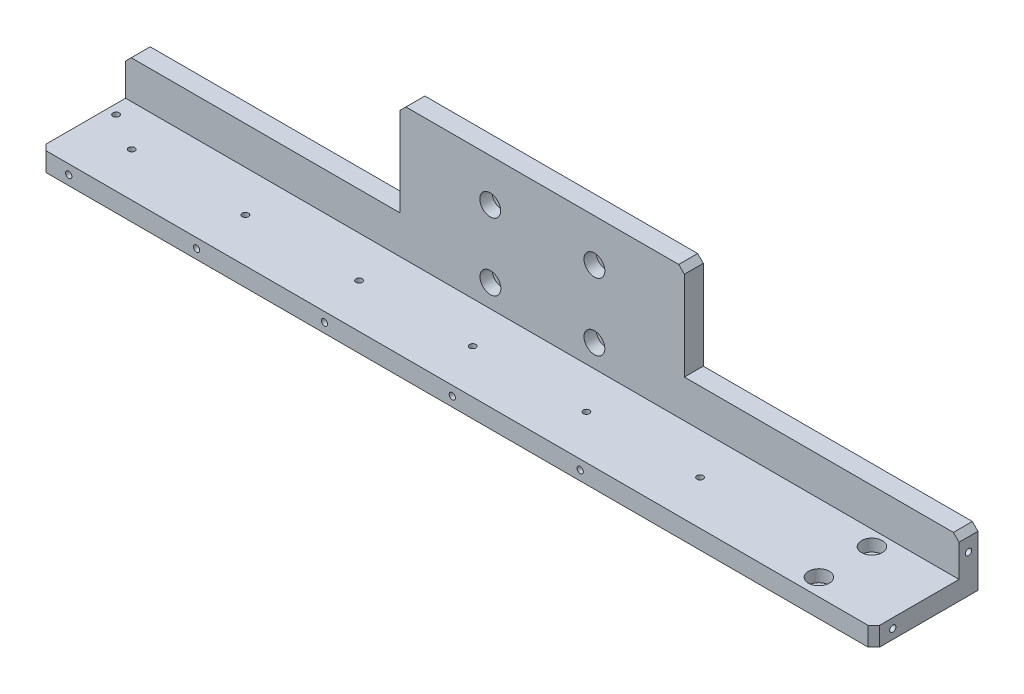
SolidWorks part; units mm, degrees
material "6061-T6"
ref_plane "前视基准面" through (0, 0, 0) normal (0, 0, 1) x (1, 0, 0)
ref_plane "上视基准面" through (0, 0, 0) normal (0, 1, 0) x (1, 0, 0)
ref_plane "右视基准面" through (0, 0, 0) normal (1, 0, 0) x (0, 0, -1)
sketch "草图2" plane through (0, 0, 0) normal (0, 0, 1) x (1, 0, 0)
  line L2 (-220, 0) -> (-220, -80)
  line L3 (-220, -80) -> (220, -80)
  line L6 (-220, 0) -> (220, 0)
  line L8 (220, 0) -> (220, -80)
  dimension "D3" = 80
  dimension "D4" = 440
extrude "凸台-拉伸1" add sketch "草图2" along normal blind 10
sketch "草图3" plane through (0, 0, 10) normal (0, 0, 1) x (1, 0, 0)
  line L0 (220, -80) -> (220, 0) construction
  line L1 (-220, -80) -> (220, -80)
  line L2 (-220, -80) -> (-220, -70)
  line L3 (-220, -70) -> (220, -70)
  line L4 (220, -80) -> (220, -70)
  dimension "D1" = 10
extrude "凸台-拉伸2" add sketch "草图3" along normal blind 45
sketch "草图5" plane through (0, 0, 10) normal (0, 0, 1) x (1, 0, 0)
  line L0 (0, 0) -> (0, -37.7713) construction
  line L1 (-220, 0) -> (-75, 0)
  line L2 (-220, 0) -> (-220, -50)
  line L3 (-220, -50) -> (-75, -50)
  line L4 (-75, 0) -> (-75, -50)
  line L5 (220, -70) -> (-220, -70) construction
  line L6 (75, 0) -> (75, -50)
  line L7 (220, -50) -> (75, -50)
  line L8 (220, 0) -> (220, -50)
  line L9 (220, 0) -> (75, 0)
  dimension "D1" = 20
  dimension "D2" = 150
extrude "切除-拉伸2" cut sketch "草图5" against normal through all
hole_wizard "M6 六角凹头螺钉的柱形沉头孔1" positions "草图6" profile "草图7" counterbore size "M6" standard "ISO"
sketch "草图6" plane through (0, 0, 10) normal (0, 0, 1) x (1, 0, 0)
  point P0 (-27.5, -22.5205)
  point P2 (27.5, -22.5205)
  point P4 (27.5, -58)
  point P6 (-27.3962, -58)
sketch "草图7" plane through (-27.5, -22.5205, 10) normal (1, 0, 0) x (0, -1, 0)
  line L0 (0, 0) -> (0, 24.2328)
  line L1 (0, 24.2328) -> (3.3, 22.25)
  line L2 (3.3, 22.25) -> (3.3, 6.4)
  line L3 (3.3, 6.4) -> (5.5, 6.4)
  line L4 (5.5, 6.4) -> (5.5, 0)
  line L5 (5.5, 0) -> (0, 0)
  line L10 (0, 24.2328) -> (-3.3, 22.25) construction
  line L11 (0, -6.35) -> (0, 107.95) construction
  dimension "孔直径" = 6.6
  dimension "孔深度" = 22.25
  dimension "柱形沉头孔直径" = 11
  dimension "柱形沉头孔深度" = 6.4
  dimension "导头角度" = 118
hole_wizard "M4 螺纹孔1" positions "草图8" profile "草图9" tap size "M4" standard "ISO"
sketch "草图8" plane through (0, -70, 0) normal (0, 1, 0) x (1, 0, 0)
  point P0 (-195, -31.7428)
  point P2 (-135, -31.7428)
  point P4 (-75, -31.7428)
  point P6 (-15, -31.7428)
  point P8 (45, -31.7428)
  point P10 (105, -31.7428)
sketch "草图9" plane through (-195, -70, 31.7428) normal (1, 0, 0) x (0, 0, 1)
  line L0 (0, 0) -> (0, 12.4914)
  line L1 (0, 12.4914) -> (1.65, 11.5)
  line L2 (1.65, 11.5) -> (1.65, 0)
  line L5 (1.65, 0) -> (0, 0)
  line L10 (0, 12.4914) -> (-1.65, 11.5) construction
  line L11 (0, -6.35) -> (0, 107.95) construction
  dimension "螺纹孔钻头直径" = 3.3
  dimension "螺纹孔钻头深度" = 11.5
  dimension "导头角度" = 118
cosmetic thread "孔螺蚊线1" parameters "D1"=8, "D2"=4
cosmetic thread "孔螺蚊线2" parameters "D1"=8, "D2"=4
cosmetic thread "孔螺蚊线3" parameters "D1"=8, "D2"=4
cosmetic thread "孔螺蚊线4" parameters "D1"=8, "D2"=4
cosmetic thread "孔螺蚊线5" parameters "D1"=8, "D2"=4
cosmetic thread "孔螺蚊线6" parameters "D1"=8, "D2"=4
hole_wizard "M4 螺纹孔2" positions "草图10" profile "草图11" tap size "M4" standard "ISO"
sketch "草图10" plane through (0, 0, 55) normal (0, 0, 1) x (1, 0, 0)
  line L0 (-220, -80) -> (220, -80) construction
  line L1 (-220, -70) -> (-220, -80) construction
  line L2 (-205, -75) -> (-137.5, -75) construction
  line L3 (-137.5, -75) -> (-70, -75) construction
  line L4 (-70, -75) -> (-2.5, -75) construction
  line L5 (-2.5, -75) -> (65, -75) construction
  point P0 (-205, -75)
  point P2 (-137.5, -75)
  point P13 (-70, -75)
  point P15 (-2.5, -75)
  point P17 (65, -75)
  dimension "D1" = 67.5
  dimension "D2" = 5
  dimension "D3" = 15
  dimension "D4" = 67.5
  dimension "D5" = 67.5
  dimension "D6" = 67.5
sketch "草图11" plane through (-205, -75, 55) normal (1, 0, 0) x (0, -1, 0)
  line L0 (0, 0) -> (0, 12.4914)
  line L1 (0, 12.4914) -> (1.65, 11.5)
  line L2 (1.65, 11.5) -> (1.65, 0)
  line L5 (1.65, 0) -> (0, 0)
  line L10 (0, 12.4914) -> (-1.65, 11.5) construction
  line L11 (0, -6.35) -> (0, 107.95) construction
  dimension "螺纹孔钻头直径" = 3.3
  dimension "螺纹孔钻头深度" = 11.5
  dimension "导头角度" = 118
cosmetic thread "孔螺蚊线7" parameters "D1"=8, "D2"=4
cosmetic thread "孔螺蚊线8" parameters "D1"=8, "D2"=4
cosmetic thread "孔螺蚊线9" parameters "D1"=8, "D2"=4
cosmetic thread "孔螺蚊线10" parameters "D1"=8, "D2"=4
cosmetic thread "孔螺蚊线11" parameters "D1"=8, "D2"=4
chamfer "倒角1" distance 3 angle 45 6 edges at (220, -75, 55) (220, -50, 5) (75, 0, 5) (-75, 0, 5) (-220, -75, 55) (-220, -50, 5)
hole_wizard "M6 六角凹头螺钉的柱形沉头孔2" positions "草图12" profile "草图13" counterbore size "M6" standard "ISO"
sketch "草图12" plane through (0, -70, 0) normal (0, 1, 0) x (1, 0, 0)
  point P0 (182, -18)
  point P2 (182, -46)
sketch "草图13" plane through (182, -70, 18) normal (1, 0, 0) x (0, 0, 1)
  line L0 (0, 0) -> (0, 18.9828)
  line L1 (0, 18.9828) -> (3.3, 17)
  line L2 (3.3, 17) -> (3.3, 6.4)
  line L3 (3.3, 6.4) -> (5.5, 6.4)
  line L4 (5.5, 6.4) -> (5.5, 0)
  line L5 (5.5, 0) -> (0, 0)
  line L10 (0, 18.9828) -> (-3.3, 17) construction
  line L11 (0, -6.35) -> (0, 107.95) construction
  dimension "孔直径" = 6.6
  dimension "孔深度" = 17
  dimension "柱形沉头孔直径" = 11
  dimension "柱形沉头孔深度" = 6.4
  dimension "导头角度" = 118
hole_wizard "M4 螺纹孔3" positions "草图14" profile "草图15" tap size "M4" standard "ISO"
sketch "草图14" plane through (0, -70, 0) normal (0, 1, 0) x (1, 0, 0)
  line L0 (-220, -52) -> (-220, -10) construction
  line L1 (220, -10) -> (-220, -10) construction
  point P0 (-215, -20)
  dimension "D1" = 5
  dimension "D2" = 10
sketch "草图15" plane through (-215, -70, 20) normal (1, 0, 0) x (0, 0, 1)
  line L0 (0, 0) -> (0, 12.4914)
  line L1 (0, 12.4914) -> (1.65, 11.5)
  line L2 (1.65, 11.5) -> (1.65, 0)
  line L5 (1.65, 0) -> (0, 0)
  line L10 (0, 12.4914) -> (-1.65, 11.5) construction
  line L11 (0, -6.35) -> (0, 107.95) construction
  dimension "螺纹孔钻头直径" = 3.3
  dimension "螺纹孔钻头深度" = 11.5
  dimension "导头角度" = 118
cosmetic thread "孔螺蚊线12" parameters "D1"=8, "D2"=4
ref_plane "基准面1" through (0, 0, 0) normal (1, 0, 0) x (0, 0, -1)
hole_wizard "M4 螺纹孔4" positions "草图16" profile "草图17" tap size "M4" standard "ISO"
sketch "草图16" plane through (-220, 0, 0) normal (-1, 0, 0) x (0, 0, 1)
  line L0 (5, -60) -> (5, -53) construction
  line L1 (10, -53) -> (0, -53) construction
  line L3 (45, -75) -> (52, -75) construction
  line L4 (52, -80) -> (52, -70) construction
  line L6 (55, -70) -> (55, -80) construction
  line L7 (0, -50) -> (10, -50) construction
  point P0 (45, -75)
  point P2 (5, -60)
  dimension "D1" = 10
  dimension "D2" = 10
sketch "草图17" plane through (-220, -75, 45) normal (0, 1, 0) x (0, 0, 1)
  line L0 (0, 0) -> (0, 12.4914)
  line L1 (0, 12.4914) -> (1.65, 11.5)
  line L2 (1.65, 11.5) -> (1.65, 0)
  line L5 (1.65, 0) -> (0, 0)
  line L10 (0, 12.4914) -> (-1.65, 11.5) construction
  line L11 (0, -6.35) -> (0, 107.95) construction
  dimension "螺纹孔钻头直径" = 3.3
  dimension "螺纹孔钻头深度" = 11.5
  dimension "导头角度" = 118
cosmetic thread "孔螺蚊线13" parameters "D1"=8, "D2"=4
cosmetic thread "孔螺蚊线14" parameters "D1"=8, "D2"=4
mirror "镜向1" about plane through (0, 0, 0) normal (1, 0, 0) of "M4 螺纹孔4"
hole_wizard "M4 螺纹孔5" positions "草图18" profile "草图19" tap size "M4" standard "ISO"
sketch "草图18" plane through (0, 0, 0) normal (0, 0, -1) x (-1, 0, 0)
  line L2 (-220, -80) -> (-220, -53) construction
  line L3 (0, -80) -> (0, -126.6785) construction
  line L4 (220, -80) -> (-220, -80) construction
  line L5 (0, 14.85) -> (0, -14.85) construction
  point P0 (-47.5, -75)
  point P18 (47.5, -75)
  dimension "D1" = 5
  dimension "D2" = 172.5
sketch "草图19" plane through (47.5, -75, 0) normal (1, 0, 0) x (0, 1, 0)
  line L0 (0, 0) -> (0, 12.4914)
  line L1 (0, 12.4914) -> (1.65, 11.5)
  line L2 (1.65, 11.5) -> (1.65, 0)
  line L5 (1.65, 0) -> (0, 0)
  line L10 (0, 12.4914) -> (-1.65, 11.5) construction
  line L11 (0, -6.35) -> (0, 107.95) construction
  dimension "螺纹孔钻头直径" = 3.3
  dimension "螺纹孔钻头深度" = 11.5
  dimension "导头角度" = 118
cosmetic thread "孔螺蚊线15" parameters "D1"=8, "D2"=4
cosmetic thread "孔螺蚊线16" parameters "D1"=8, "D2"=4
